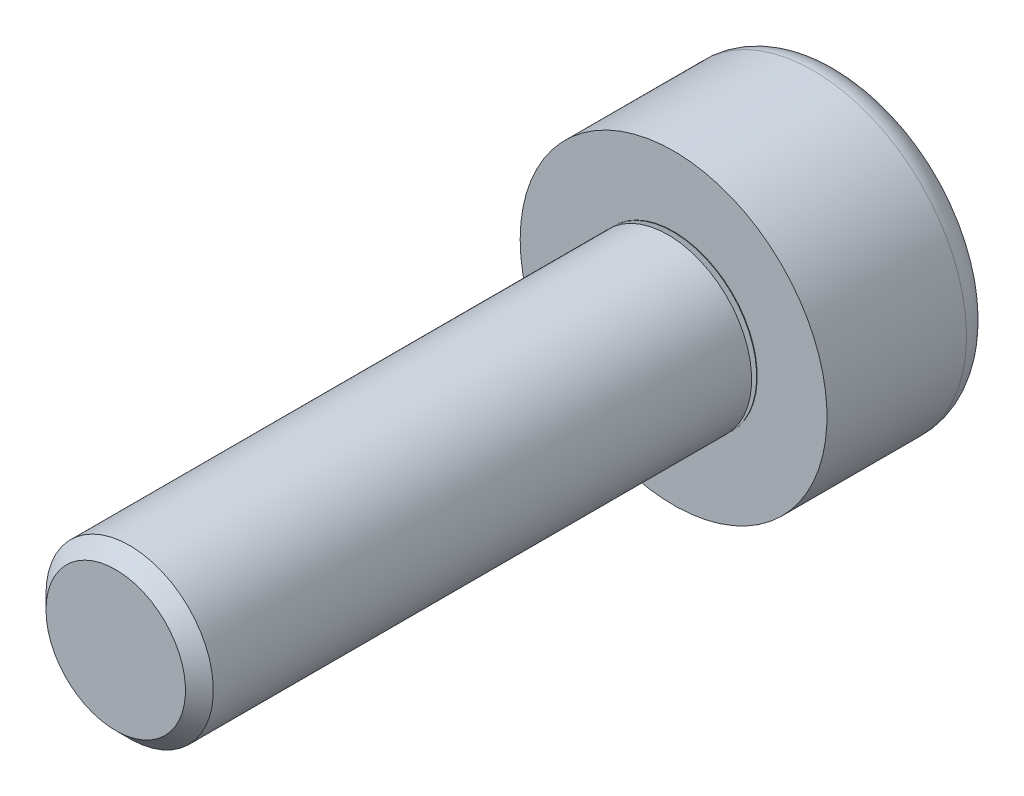
SolidWorks part; units mm, degrees
ref_plane "Front" through (0, 0, 0) normal (0, 0, 1) x (1, 0, 0)
ref_plane "Top" through (0, 0, 0) normal (0, 1, 0) x (1, 0, 0)
ref_plane "Right" through (0, 0, 0) normal (1, 0, 0) x (0, 0, -1)
sketch "Logo3_Revol_Axis" plane through (0, 0, 0) normal (0, 1, 0) x (1, 0, 0)
  line L0 (0, -43.5172) -> (0, 43.5172) construction
sketch "Logo3_bib1" plane through (0, 0, 0) normal (0, -1, 0) x (-1, 0, 0)
  line L0 (0, -10) -> (0, 3)
  line L1 (0, 3) -> (2.25, 3)
  line L2 (2.75, 2.5) -> (2.75, 0)
  line L3 (2.75, 0) -> (1.5, 0)
  line L4 (1.5, 0) -> (1.5, -0.01)
  line L5 (1.5, -9.75) -> (1.25, -10)
  line L6 (1.25, -10) -> (0, -10)
  line L7 (1.5, -0.01) -> (1.3634, -0.01)
  line L8 (1.3566, -0.0488) -> (1.5, -0.101)
  line L9 (1.5, -0.101) -> (1.5, -9.75)
  line L10 (0, 10.5852) -> (0, -63.2873) construction
  arc A0 (2.25, 3) -> (2.75, 2.5) centre (2.25, 2.5) cw
  arc A1 (1.3634, -0.01) -> (1.3566, -0.0488) centre (1.3634, -0.03) ccw
  point P17 (1.25, -0.01)
revolve "Revolve1" add sketch "Logo3_bib1" angle 360 about L10
cosmetic thread "Cosmetic Thread1" parameters "D2"=2.5
sketch "Logo3_bib2" plane through (0, 0, -3) normal (0, 0, -1) x (1, 0, 0)
  line L1 (1.4434, 0) -> (0.7217, 1.25)
  line L2 (0.7217, 1.25) -> (-0.7217, 1.25)
  line L3 (-0.7217, 1.25) -> (-1.4434, 0)
  line L4 (-1.4434, 0) -> (-0.7217, -1.25)
  line L5 (-0.7217, -1.25) -> (0.7217, -1.25)
  line L6 (0.7217, -1.25) -> (1.4434, 0)
  circle A0 centre (0, 0) radius 1.25 construction
extrude "Cut-Extrude1" cut sketch "Logo3_bib2" against normal blind 1.25
equation "\"DIA2@XZQB7_bib1\" = \"XZQB7_d1-pas@XZQB7_bib1\""
equation "\"LGT1@XZQB7_bib1\" = \"XZQB7_d1@XZQB7_bib1\""
equation "\"D1@Cut-Extrude1\" = \"XZQB7_c1@XZQB7_bib2\"/2."
equation "\"D2@Cosmetic Thread1\" = \"XZQB7_d1-pas@XZQB7_bib1\""
